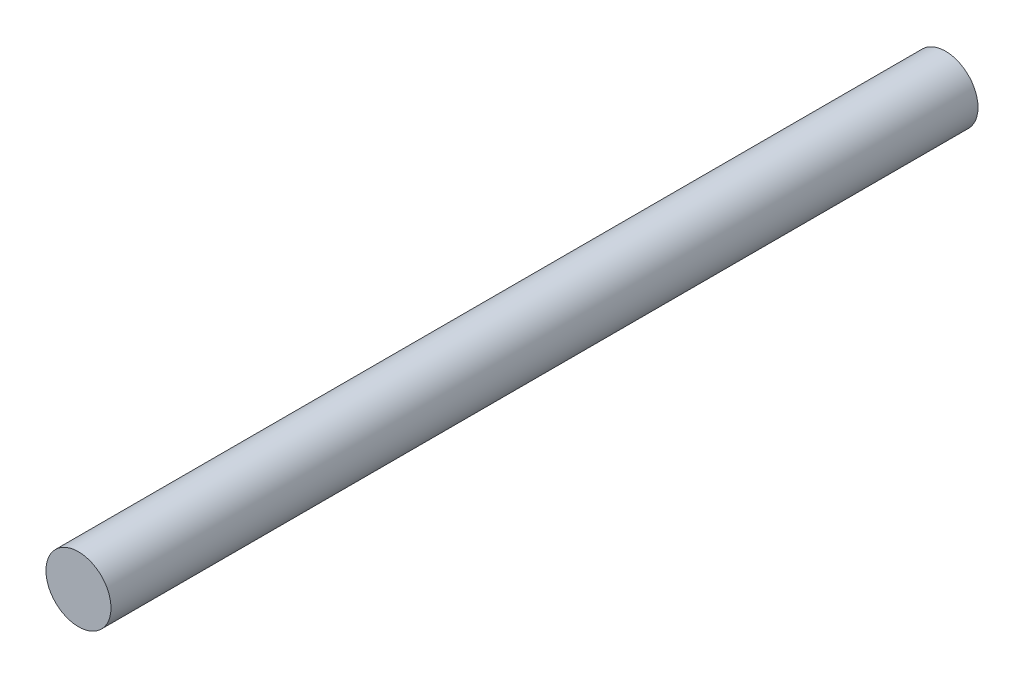
SolidWorks part; units mm, degrees
material "S45C"
ref_plane "前视基准面" through (0, 0, 0) normal (0, 0, 1) x (1, 0, 0)
ref_plane "上视基准面" through (0, 0, 0) normal (0, 1, 0) x (1, 0, 0)
ref_plane "右视基准面" through (0, 0, 0) normal (1, 0, 0) x (0, 0, -1)
sketch "草图1" plane through (0, 0, 0) normal (0, 0, 1) x (1, 0, 0)
  circle A0 centre (0, 0) radius 3
  dimension "D1" = 6
extrude "凸台-拉伸1" add sketch "草图1" along normal blind 80
